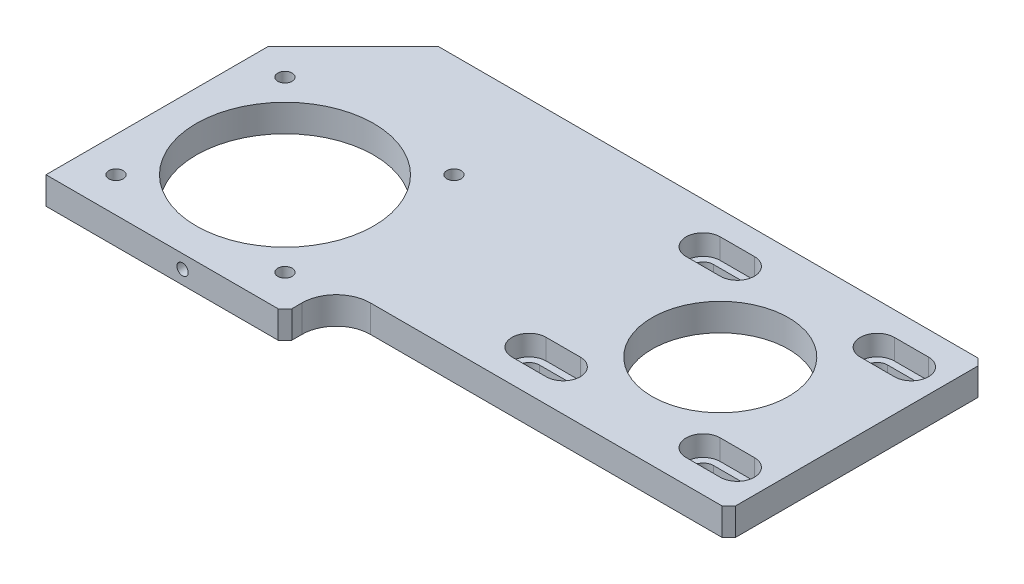
from build123d import *

# Parameters (mm, degrees)
SKETCH_2_W             = 185
SKETCH_2_H             = 90
EXTRUDE_1_DEPTH        = 8
SKETCH_4_W             = 115
SKETCH_4_H             = 15
CUT_EXTRUDE_7_DEPTH    = 104.175820811
SKETCH_5_R             = 26
CUT_EXTRUDE_8_DEPTH    = 104.175820811
HOLE_WIZARD_M5_1_D     = 4.2
SKETCH_10_R            = 20
CUT_EXTRUDE_9_DEPTH    = 104.175820811
CUT_EXTRUDE_15_DEPTH   = 6
CUT_EXTRUDE_16_DEPTH   = 104.040040761
HOLE_WIZARD_M4_1_D     = 3.3
HOLE_WIZARD_M4_1_DEPTH = 12
HOLE_WIZARD_M4_1_TIP   = 0.991420021
HOLE_WIZARD_M4_2_D     = 3.3
HOLE_WIZARD_M4_2_DEPTH = 12
HOLE_WIZARD_M4_2_TIP   = 0.991420021
CHAMFER_1_SIZE         = 25
CHAMFER_2_SIZE         = 2
FILLET_1_R             = 10


with BuildPart() as part:
    # 草图2 → 凸台-拉伸1 (new body)
    with BuildSketch(Plane(origin=(0, 0, 0), x_dir=(1, 0, 0), z_dir=(0, 1, 0))):
        Rectangle(SKETCH_2_W, SKETCH_2_H)
    extrude(amount=EXTRUDE_1_DEPTH)

    # 草图4 → 切除-拉伸7 (cut, through all)
    with BuildSketch(Plane(origin=(0, 8, 0), x_dir=(1, 0, 0), z_dir=(0, 1, 0))):
        with Locations((35, -37.5)):
            Rectangle(SKETCH_4_W, SKETCH_4_H)
    extrude(amount=-CUT_EXTRUDE_7_DEPTH, mode=Mode.SUBTRACT)

    # 草图5 → 切除-拉伸8 (cut, through all)
    with BuildSketch(Plane(origin=(0, 8, 0), x_dir=(1, 0, 0), z_dir=(0, 1, 0))):
        with Locations(Location((-57.5, -10, 0), (0, 0, 270))):
            Circle(SKETCH_5_R)
    extrude(amount=-CUT_EXTRUDE_8_DEPTH, mode=Mode.SUBTRACT)

    # M5 螺纹孔1 (through all)
    with Locations(Plane(origin=(0, 8, 0), x_dir=(1, 0, 0), z_dir=(0, 1, 0))):
        with Locations((-82.248737342, 14.748737342), (-32.751262658, 14.748737342), (-32.751262658, -34.748737342), (-82.248737342, -34.748737342), (-57.5, -10)):
            Hole(HOLE_WIZARD_M5_1_D / 2)

    # 草图10 → 切除-拉伸9 (cut, through all)
    with BuildSketch(Plane(origin=(0, 8, 0), x_dir=(1, 0, 0), z_dir=(0, 1, 0))):
        with Locations(Location((52.5, 7.5, 0), (0, 0, 270))):
            Circle(SKETCH_10_R)
    extrude(amount=-CUT_EXTRUDE_9_DEPTH, mode=Mode.SUBTRACT)

    # 草图15 → 切除-拉伸15 (cut)
    with BuildSketch(Plane(origin=(0, 8, 0), x_dir=(1, 0, 0), z_dir=(0, 1, 0))):
        with BuildLine():
            Line((73, -13), (83, -13))
            ThreePointArc((83, -13), (88, -18), (83, -23))
            Line((83, -23), (73, -23))
            ThreePointArc((73, -23), (68, -18), (73, -13))
        make_face()
        with BuildLine():
            Line((73, 28), (83, 28))
            ThreePointArc((83, 28), (88, 33), (83, 38))
            Line((83, 38), (73, 38))
            ThreePointArc((73, 38), (68, 33), (73, 28))
        make_face()
        with BuildLine():
            Line((22, -13), (32, -13))
            ThreePointArc((32, -13), (37, -18), (32, -23))
            Line((32, -23), (22, -23))
            ThreePointArc((22, -23), (17, -18), (22, -13))
        make_face()
        with BuildLine():
            Line((22, 28), (32, 28))
            ThreePointArc((32, 28), (37, 33), (32, 38))
            Line((32, 38), (22, 38))
            ThreePointArc((22, 38), (17, 33), (22, 28))
        make_face()
    extrude(amount=-CUT_EXTRUDE_15_DEPTH, mode=Mode.SUBTRACT)

    # 草图16 → 切除-拉伸16 (cut, through all)
    with BuildSketch(Plane(origin=(0, 2, 0), x_dir=(1, 0, 0), z_dir=(0, 1, 0))):
        with BuildLine():
            Line((73, -15), (83, -15))
            ThreePointArc((83, -15), (86, -18), (83, -21))
            Line((83, -21), (73, -21))
            ThreePointArc((73, -21), (70, -18), (73, -15))
        make_face()
        with BuildLine():
            Line((73, 30), (83, 30))
            ThreePointArc((83, 30), (86, 33), (83, 36))
            Line((83, 36), (73, 36))
            ThreePointArc((73, 36), (70, 33), (73, 30))
        make_face()
        with BuildLine():
            Line((22, -15), (32, -15))
            ThreePointArc((32, -15), (35, -18), (32, -21))
            Line((32, -21), (22, -21))
            ThreePointArc((22, -21), (19, -18), (22, -15))
        make_face()
        with BuildLine():
            Line((22, 30), (32, 30))
            ThreePointArc((32, 30), (35, 33), (32, 36))
            Line((32, 36), (22, 36))
            ThreePointArc((22, 36), (19, 33), (22, 30))
        make_face()
    extrude(amount=-CUT_EXTRUDE_16_DEPTH, mode=Mode.SUBTRACT)

    # M4 螺纹孔1
    with Locations(Plane(origin=(0, 0, -45), x_dir=(-1, 0, 0), z_dir=(0, 0, -1))):
        with Locations((-52.5, 4), (52.5, 4)):
            Hole(HOLE_WIZARD_M4_1_D / 2, depth=HOLE_WIZARD_M4_1_DEPTH)
            with Locations((0, 0, -(HOLE_WIZARD_M4_1_DEPTH + HOLE_WIZARD_M4_1_TIP / 2))):  # 118° drill point
                Cone(0, HOLE_WIZARD_M4_1_D / 2, HOLE_WIZARD_M4_1_TIP, mode=Mode.SUBTRACT)

    # M4 螺纹孔2
    with Locations(Plane.XY.offset(45)):
        with Locations((-52.5, 4)):
            Hole(HOLE_WIZARD_M4_2_D / 2, depth=HOLE_WIZARD_M4_2_DEPTH)
            with Locations((0, 0, -(HOLE_WIZARD_M4_2_DEPTH + HOLE_WIZARD_M4_2_TIP / 2))):  # 118° drill point
                Cone(0, HOLE_WIZARD_M4_2_D / 2, HOLE_WIZARD_M4_2_TIP, mode=Mode.SUBTRACT)

    # 倒角1
    chamfer_1_edges = [part.edges().sort_by_distance(p)[0] for p in [
        (-92.5, 4, -45),
    ]]
    chamfer(chamfer_1_edges, length=CHAMFER_1_SIZE)

    # 倒角2
    chamfer_2_edges = [part.edges().sort_by_distance(p)[0] for p in [
        (92.5, 4, 30),
        (-22.5, 4, 45),
        (92.5, 4, -45),
    ]]
    chamfer(chamfer_2_edges, length=CHAMFER_2_SIZE)

    # 圆角1
    fillet_1_edges = [part.edges().sort_by_distance(p)[0] for p in [
        (-22.5, 4, 30),
    ]]
    fillet(fillet_1_edges, radius=FILLET_1_R)


solid = part.part
